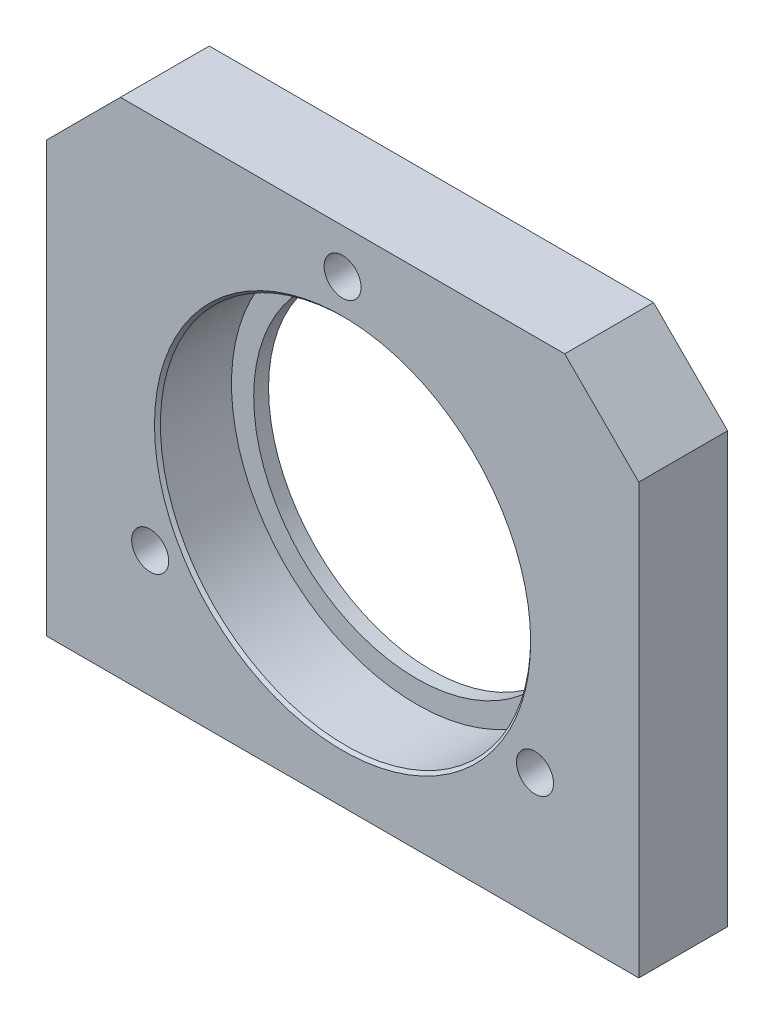
SolidWorks part; units mm, degrees
ref_plane "前视基准面" through (0, 0, 0) normal (0, 0, 1) x (1, 0, 0)
ref_plane "上视基准面" through (0, 0, 0) normal (0, 1, 0) x (1, 0, 0)
ref_plane "右视基准面" through (0, 0, 0) normal (1, 0, 0) x (0, 0, -1)
sketch "草图1" plane through (0, 0, 0) normal (0, 0, 1) x (1, 0, 0)
  line L0 (-78.3813, 0) -> (76.5587, 0) construction
  line L1 (0, 68.0357) -> (0, -86.1786) construction
  line L2 (-20, -16) -> (20, -16)
  line L3 (-15, 18) -> (15, 18)
  line L4 (-20, 13) -> (-20, -16)
  line L5 (20, 13) -> (20, -16)
  line L6 (-20, 13) -> (-15, 18)
  line L7 (-78.3813, 18) -> (76.5587, 18) construction
  line L8 (-20, 68.0357) -> (-20, -86.1786) construction
  line L9 (20, 68.0357) -> (20, -86.1786) construction
  line L10 (-78.3813, -16) -> (76.5587, -16) construction
  line L11 (15, 18) -> (20, 13)
  circle A0 centre (0, 0) radius 11
  point P13 (-20, 18)
  point P14 (20, 18)
  dimension "D5" = 22
  dimension "D1" = 16
  dimension "D2" = 34
  dimension "D3" = 20
  dimension "D4" = 20
extrude "凸台-拉伸1" add sketch "草图1" along normal blind 6
sketch "草图2" plane through (0, 0, 6) normal (0, 0, 1) x (1, 0, 0)
  circle A0 centre (0, 0) radius 12.5
  dimension "D1" = 25
extrude "切除-拉伸1" cut sketch "草图2" against normal blind 5
sketch "草图3" plane through (0, 0, 6) normal (0, 0, 1) x (1, 0, 0)
  line L0 (0, 19.6942) -> (0, -18.245) construction
  line L1 (-24.4436, 0) -> (27.0601, 0) construction
  line L2 (0, 0) -> (-19.8521, -11.4616) construction
  line L3 (0, 0) -> (23.6318, -13.6438) construction
  circle A0 centre (0, 0) radius 15 construction
  dimension "D1" = 30
  dimension "D2" = 120
  dimension "D3" = 120
hole_wizard "M3 螺纹孔1" positions "3D草图2" profile "草图5" tap size "M3" standard "GB" end condition through all
sketch3d "3D草图2"
  line L0 (0, 19.6942, 6) -> (0, -18.245, 6) construction
  line L1 (0, 0, 6) -> (-19.8521, -11.4616, 6) construction
  line L2 (0, 0, 6) -> (23.6318, -13.6438, 6) construction
  circle A0 centre (0, 0, 6) radius 15 construction
  point P0 (0, 15.0056, 6)
  point P4 (-12.9904, -7.5, 6)
  point P10 (0, 0, 21)
  point P11 (12.9904, -7.5, 6)
sketch "草图5" plane through (0, 15.0056, 6) normal (1, 0, 0) x (0, -1, 0)
  line L0 (0, 0) -> (0, 6)
  line L1 (0, 6) -> (1.25, 6)
  line L2 (1.25, 6) -> (1.25, 0)
  line L5 (1.25, 0) -> (0, 0)
  line L11 (0, -6.35) -> (0, 107.95) construction
  dimension "通孔螺纹孔钻头直径" = 2.5
  dimension "通孔螺纹孔钻头深度" = 6
cosmetic thread "孔螺蚊线1" parameters "D2"=3
cosmetic thread "孔螺蚊线2" parameters "D2"=3
cosmetic thread "孔螺蚊线3" parameters "D2"=3
sketch "草图6" plane through (0, -16, 0) normal (0, -1, 0) x (1, 0, 0)
  line L0 (0, -9.4252) -> (0, 15.0497) construction
  line L1 (16, -9.4252) -> (16, 15.0497) construction
  line L2 (-16, -9.4252) -> (-16, 15.0497) construction
  line L3 (-23.4344, 3) -> (28.1705, 3) construction
  dimension "D1" = 16
  dimension "D2" = 16
hole_wizard "M3 螺纹孔2" positions "3D草图3" profile "草图7" tap size "M3" standard "GB"
sketch3d "3D草图3"
  line L0 (-16, -16, -9.4252) -> (-16, -16, 15.0497) construction
  line L1 (-23.4344, -16, 3) -> (28.1705, -16, 3) construction
  line L2 (16, -16, -9.4252) -> (16, -16, 15.0497) construction
  point P0 (-16, -16, 3)
  point P6 (16, -16, 3)
sketch "草图7" plane through (-16, -16, 3) normal (1, 0, 0) x (0, 0, -1)
  line L0 (0, 0) -> (0, 6.7511)
  line L1 (0, 6.7511) -> (1.25, 6)
  line L2 (1.25, 6) -> (1.25, 0)
  line L5 (1.25, 0) -> (0, 0)
  line L10 (0, 6.7511) -> (-1.25, 6) construction
  line L11 (0, -6.35) -> (0, 107.95) construction
  dimension "螺纹孔钻头直径" = 2.5
  dimension "螺纹孔钻头深度" = 6
  dimension "导头角度" = 118
cosmetic thread "孔螺蚊线4" parameters "D1"=6, "D2"=3
cosmetic thread "孔螺蚊线5" parameters "D1"=6, "D2"=3
chamfer "倒角1" distance 0.2 angle 45 1 edges at (12.5, 0, 6)
